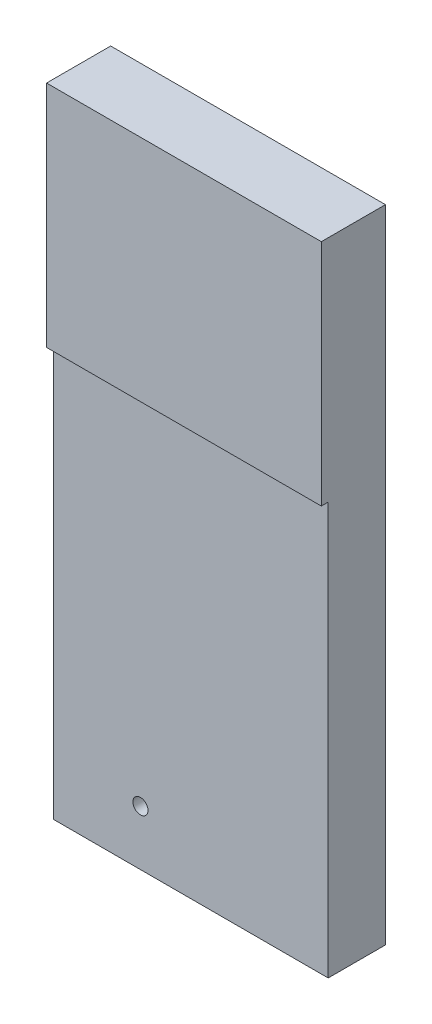
SolidWorks part; units mm, degrees
ref_plane "前视基准面" through (0, 0, 0) normal (0, 0, 1) x (1, 0, 0)
ref_plane "上视基准面" through (0, 0, 0) normal (0, 1, 0) x (1, 0, 0)
ref_plane "右视基准面" through (0, 0, 0) normal (1, 0, 0) x (0, 0, -1)
sketch "草图1" plane through (0, 0, 0) normal (0, 0, 1) x (1, 0, 0)
  line L1 (-30, -70) -> (30, -70)
  line L2 (-30, -70) -> (-30, 70)
  line L3 (-30, 70) -> (30, 70)
  line L4 (30, -70) -> (30, 70)
  line L5 (-30, -70) -> (30, 70) construction
  line L6 (-30, 70) -> (30, -70) construction
  point P0 (0, 0)
  dimension "D1" = 60
  dimension "D2" = 140
extrude "凸台-拉伸1" add sketch "草图1" along normal blind 14
sketch "草图2" plane through (0, 0, 14) normal (0, 0, 1) x (1, 0, 0)
  line L0 (30, -70) -> (30, 70) construction
  line L1 (-30, -70) -> (30, -70)
  line L2 (-30, -70) -> (-30, 20)
  line L3 (-30, 20) -> (30, 20)
  line L4 (30, -70) -> (30, 20)
  dimension "D1" = 90
extrude "切除-拉伸1" cut sketch "草图2" against normal blind 1.5
sketch "草图3" plane through (0, 0, 14) normal (0, 0, -1) x (-1, 0, 0)
  line L0 (-25, 70) -> (-25, 20)
  line L1 (-30, 70) -> (30, 70) construction
  line L2 (-30, -10) -> (30, -10)
  line L3 (35, 20) -> (35, 70)
  line L4 (35, 70) -> (-25, 70)
  line L5 (35, 20) -> (30, 20)
  line L7 (-30, -70) -> (-30, 70) construction
  line L8 (30, 70) -> (30, -70) construction
  line L9 (30, 20) -> (30, -10)
  line L10 (-25, 20) -> (-30, 20)
  line L11 (-30, 20) -> (-30, 70) construction
  line L12 (-30, 20) -> (-30, -10)
  dimension "D4" = 80
  dimension "D1" = 5
  dimension "D3" = 60
  dimension "D5" = 30
extrude "切除-拉伸2" [suppressed] cut sketch "草图3" along normal blind 1.5
hole_wizard "M4 螺纹孔1" positions "草图5" profile "草图4" tap size "M4" standard "GB" end condition through all
sketch "草图5" plane through (0, 0, 0) normal (0, 0, -1) x (-1, 0, 0)
  line L0 (30, -70) -> (-30, -70) construction
  line L2 (30, 70) -> (30, -70) construction
  point P1 (11, -58)
  dimension "D1" = 12
  dimension "D2" = 19
sketch "草图4" plane through (-11, -58, 0) normal (1, 0, 0) x (0, 1, 0)
  line L0 (0, 0) -> (0, 14)
  line L1 (0, 14) -> (1.65, 14)
  line L2 (1.65, 14) -> (1.65, 0)
  line L5 (1.65, 0) -> (0, 0)
  line L11 (0, -6.35) -> (0, 107.95) construction
  dimension "通孔螺纹孔钻头直径" = 3.3
  dimension "通孔螺纹孔钻头深度" = 14
cosmetic thread "孔螺蚊线1"
sketch "草图6" plane through (0, 0, 0) normal (0, 0, -1) x (-1, 0, 0)
  line L0 (30, -24) -> (22, -24)
  line L1 (30, 70) -> (30, -70) construction
  line L2 (22, -24) -> (22, -42)
  line L3 (22, -42) -> (30, -42)
  line L4 (30, -42) -> (30, -24)
  line L5 (30, -70) -> (-30, -70) construction
  dimension "D1" = 18
  dimension "D2" = 28
  dimension "D3" = 8
extrude "切除-拉伸3" [suppressed] cut sketch "草图6" against normal up to next
fillet "圆角1" [suppressed] radius 2
